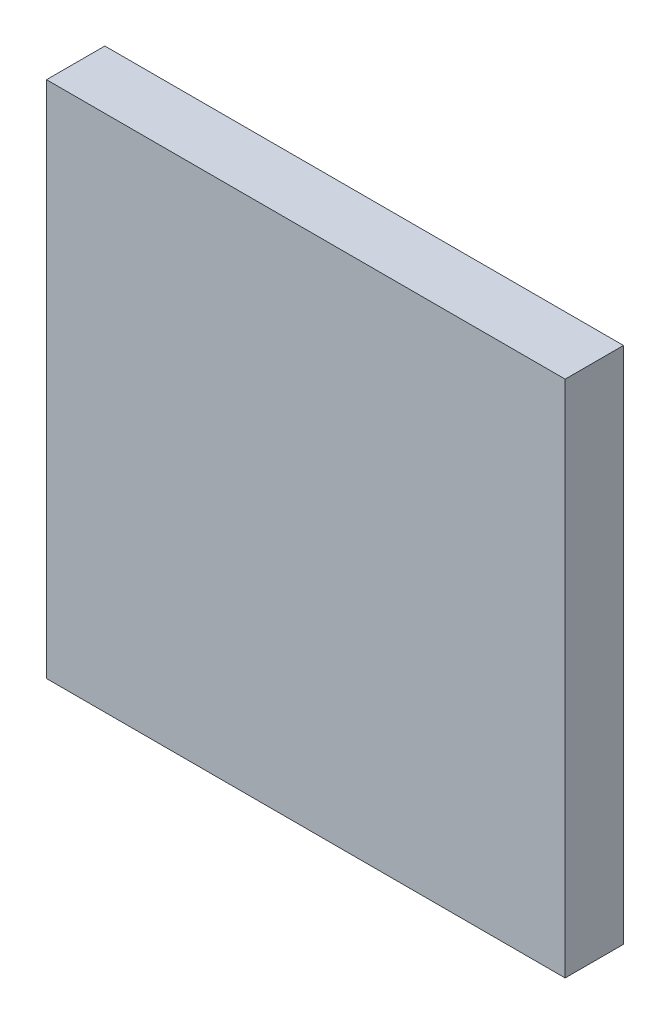
from build123d import *

# Parameters (mm, degrees)
SKETCH1_W           = 88.9
SKETCH1_H           = 88.9
BOSS_EXTRUDE1_DEPTH = 5


with BuildPart() as part:
    # Sketch1 → Boss-Extrude1 (new, symmetric)
    with BuildSketch(Plane.XY):
        Rectangle(SKETCH1_W, SKETCH1_H)
    extrude(amount=BOSS_EXTRUDE1_DEPTH, both=True)


solid = part.part
